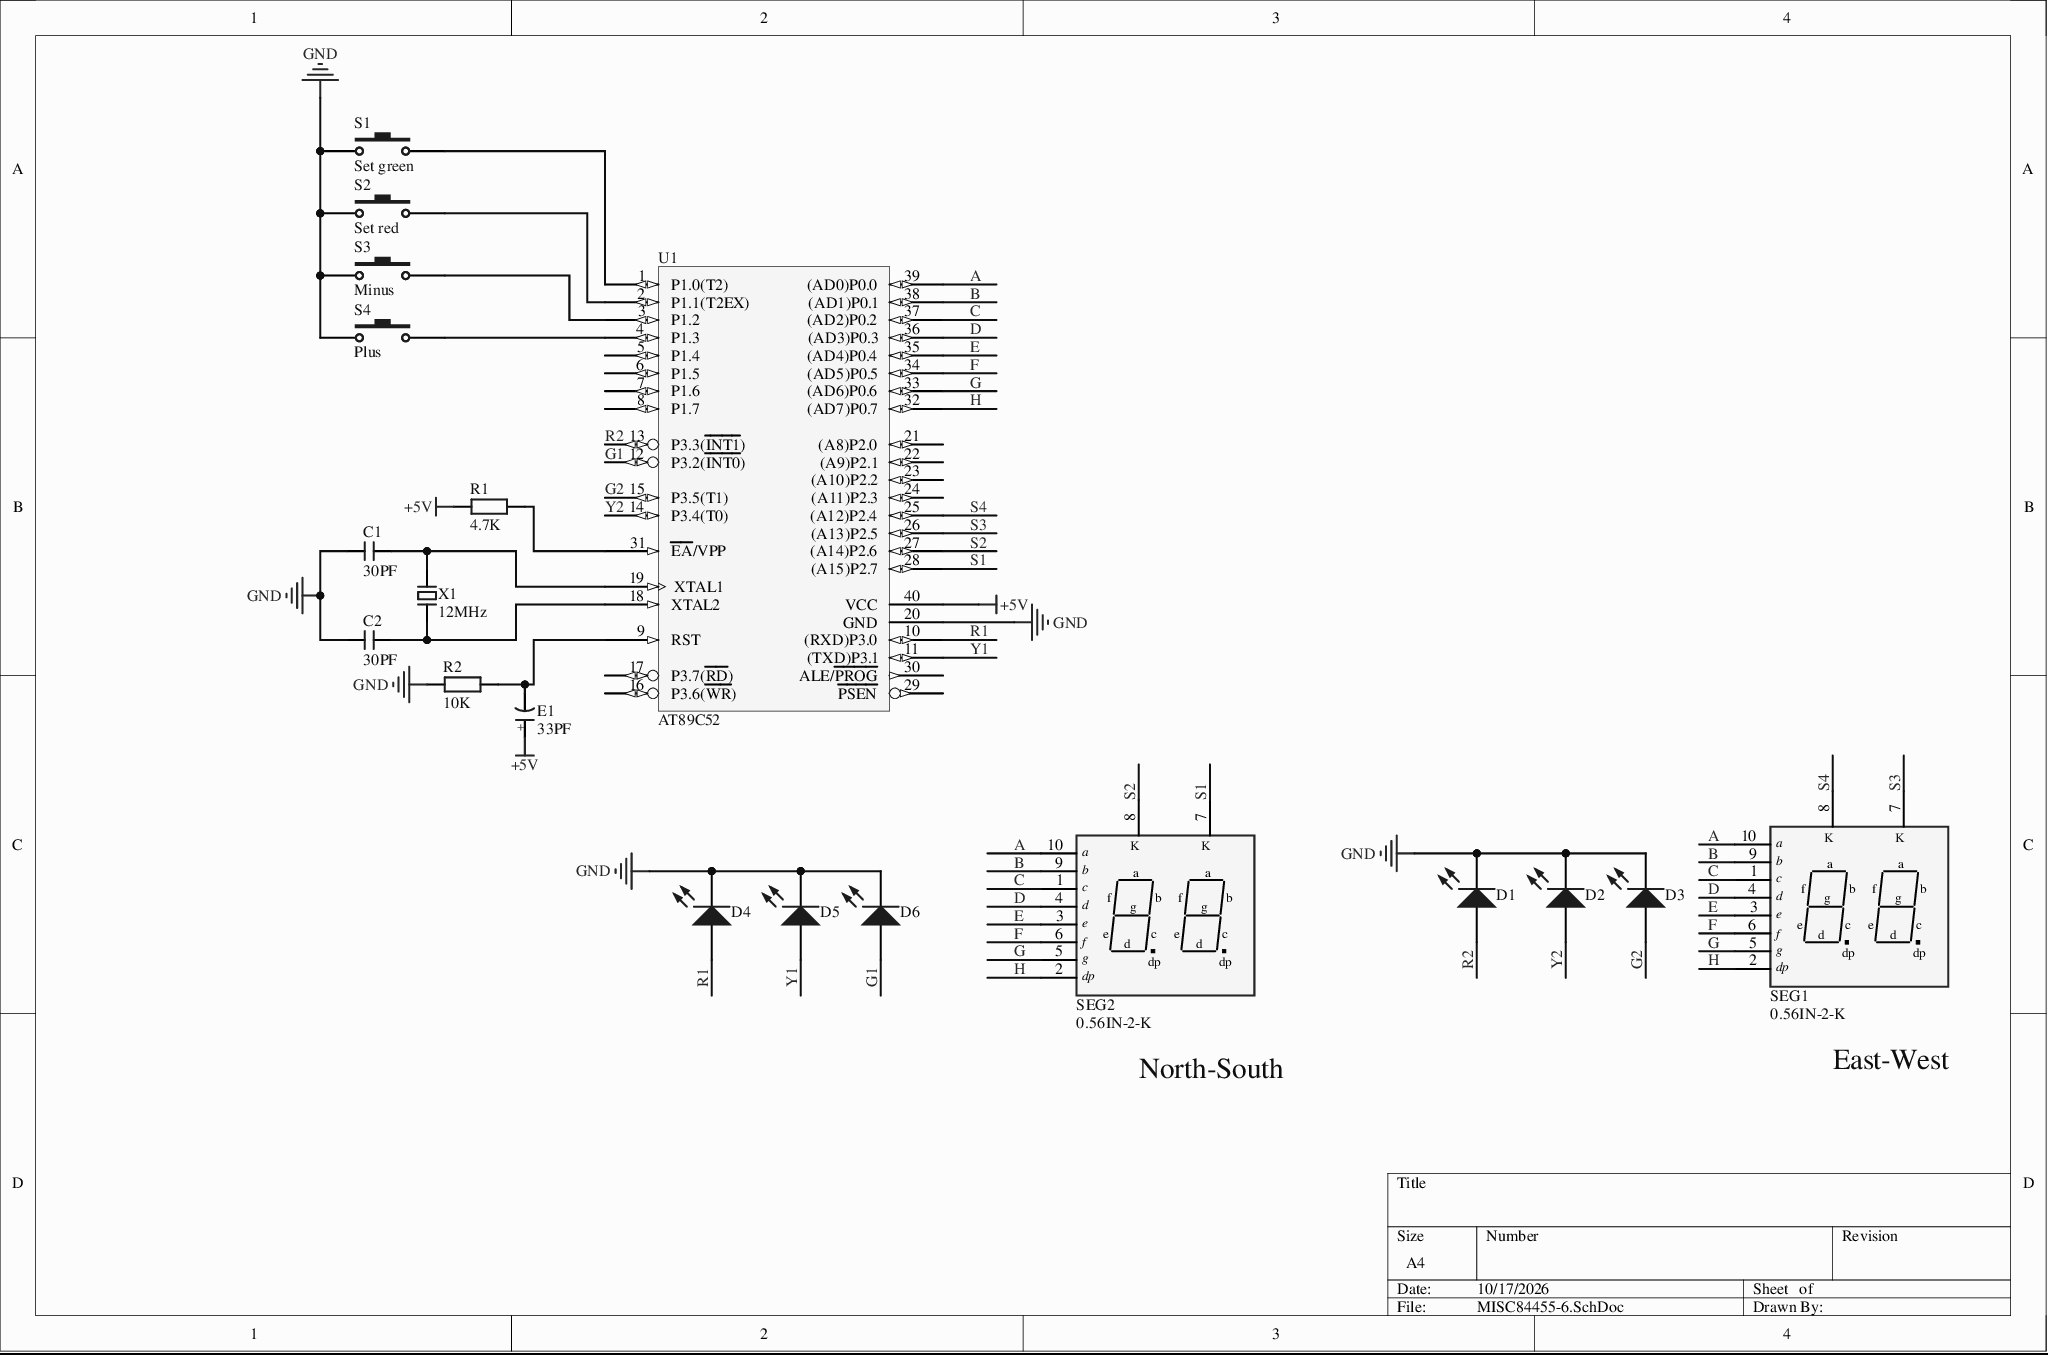
[diagram p0: MISC84455-6.SchDoc]
# Altium project MISC84455-2.PrjPcb
1 sheet, 19 parts. Net scope: global (net labels, ports and power ports of the same name join across sheets).
Board file: MISC84455.PcbDoc

## Sheet MISC84455-6.SchDoc
size A4

### Parts
C1  30PF  [CC 1.8*3.6]
C2  30PF  [CC 1.8*3.6]
D1  LED  [LED 5MM-W]  (value not drawn)
D2  LED  [LED 5MM-W]  (value not drawn)
D3  LED  [LED 5MM-W]  (value not drawn)
D4  LED  [LED 5MM-W]  (value not drawn)
D5  LED  [LED 5MM-W]  (value not drawn)
D6  LED  [LED 5MM-W]  (value not drawn)
E1  33PF  [CS 2.0*5*8 - C]
R1  4.7K  [RS 1/4W]
R2  10K  [RS 1/4W]
S1  Set green  [四脚轻触开关]
S2  Set red  [四脚轻触开关]
S3  Minus  [四脚轻触开关]
S4  Plus  [四脚轻触开关]
SEG1  0.56IN-2-K  [0.56IN-2P]
SEG2  0.56IN-2-K  [0.56IN-2P]
U1  AT89C52  [DIP40]
X1  12MHz  [OSC HC-49S]

### Nets
+5V: E1.1(A) R1.1 U1.40(VCC)
GND: C1.1 C2.1 D1.2(K) D2.2(K) D3.2(K) D4.2(K) D5.2(K) D6.2(K) R2.1 S1.1 S2.1 S3.1 S4.1 U1.20(GND)
A: SEG1.10 SEG2.10 U1.39((AD0)P0.0)
B: SEG1.9 SEG2.9 U1.38((AD1)P0.1)
C: SEG1.1 SEG2.1 U1.37((AD2)P0.2)
D: SEG1.4 SEG2.4 U1.36((AD3)P0.3)
E: SEG1.3 SEG2.3 U1.35((AD4)P0.4)
F: SEG1.6 SEG2.6 U1.34((AD5)P0.5)
G: SEG1.5 SEG2.5 U1.33((AD6)P0.6)
G1: D6.1(A) U1.12(P3.2(~{INT0}))
G2: D3.1(A) U1.15(P3.5(T1))
H: SEG1.2 SEG2.2 U1.32((AD7)P0.7)
R1: D4.1(A) U1.10((RXD)P3.0)
R2: D1.1(A) U1.13(P3.3(~{INT1}))
S1: SEG2.7 U1.28((A15)P2.7)
S2: SEG2.8 U1.27((A14)P2.6)
S3: SEG1.7 U1.26((A13)P2.5)
S4: SEG1.8 U1.25((A12)P2.4)
Y1: D5.1(A) U1.11((TXD)P3.1)
Y2: D2.1(A) U1.14(P3.4(T0))
NetC1_2: C1.2 U1.19(XTAL1) X1.2
NetC2_2: C2.2 U1.18(XTAL2) X1.1
NetE1_2: E1.2(K) R2.2 U1.9(RST)
NetR1_2: R1.2 U1.31(~{EA}/VPP)
NetS1_2: S1.2 U1.1(P1.0(T2))
NetS2_2: S2.2 U1.2(P1.1(T2EX))
NetS3_2: S3.2 U1.3(P1.2)
NetS4_2: S4.2 U1.4(P1.3)

Not connected (* = marked no-connect by the designer): U1 5(P1.4) 6(P1.5) 7(P1.6) 8(P1.7) 16(P3.6(~{WR})) 17(P3.7(~{RD})) 21((A8)P2.0) 22((A9)P2.1) 23((A10)P2.2) 24((A11)P2.3) 29(~{PSEN}) 30(ALE/~{PROG})

### Notes on the sheet
- North-South
- East-West

### Library data of the parts
C1 C2 = CC: ceramic disc capacitor; BOM名称: Through-hole ceramic disc capacitor
D1-D6 = LED: light-emitting diode
E1 = CS: through-hole solid-state capacitor; BOM名称: through-hole solid-state capacitor
R1 R2 = R-S: colour-band resistor; BOM名称: colour-band resistor
S1-S4 = SW-PB: Switch; Published: 24-Mar-1999; LatestRevisionDate: 17-Jul-2002; LatestRevisionNote: Re-released for DXP Platform.; PackageReference: SPST-2; PackageDescription: Switch; 2 Leads; Publisher: Altium Limited
SEG1 SEG2 = 0.56IN-2-K: 2-digit 0.56 inch common-cathode display
U1 = STC89C52
X1 = XTAL-2P: 2-pin passive crystal oscillator; BOM名称: 2-pin passive crystal oscillator